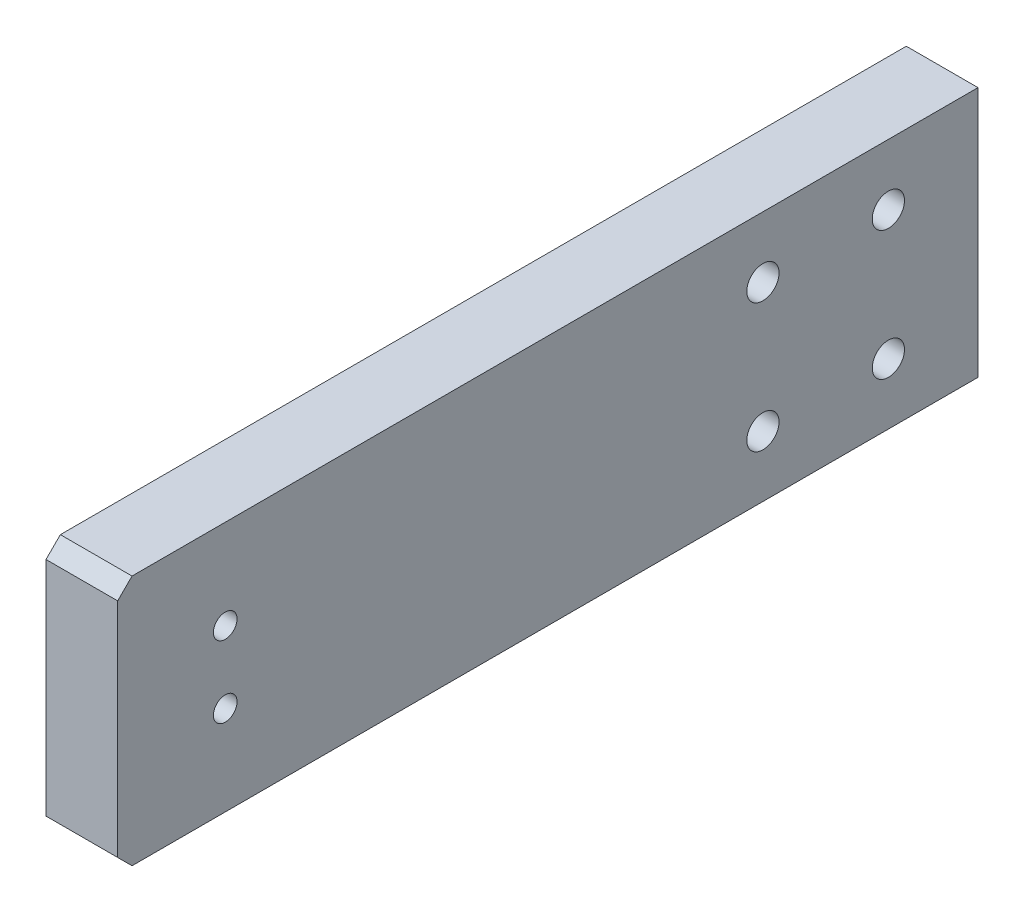
from build123d import *

# Parameters (mm, degrees)
SKETCH_1_W             = 120
SKETCH_1_H             = 35
EXTRUDE_1_DEPTH        = 10
HOLE_WIZARD_M4_1_D     = 3.3
SKETCH_5_R             = 2.25
CUT_EXTRUDE_1_DEPTH    = 28
CHAMFER_1_SIZE         = 2
PATTERN_LINEAR_1_COUNT = 2
PATTERN_LINEAR_1_PITCH = 17.5


with BuildPart() as part:
    # 草图1 → 凸台-拉伸1 (new body)
    with BuildSketch(Plane(origin=(0, 0, 0), x_dir=(0, 0, -1), z_dir=(1, 0, 0))):
        Rectangle(SKETCH_1_W, SKETCH_1_H)
    extrude(amount=EXTRUDE_1_DEPTH)

    # M4 螺纹孔1 (through all)
    with Locations(Plane.ZY):
        with Locations((45, 5), (45, -5)):
            Hole(HOLE_WIZARD_M4_1_D / 2)

    # 草图5 → 切除-拉伸1 (cut)
    with BuildSketch(Plane.ZY):
        with Locations((-47.5, 9)):
            Circle(SKETCH_5_R)
        with Locations(Location((-47.5, -9, 0), (0, 0, 180))):
            Circle(SKETCH_5_R)
    cut_extrude_1 = extrude(amount=-CUT_EXTRUDE_1_DEPTH, mode=Mode.SUBTRACT)

    # 倒角1
    chamfer_1_edges = [part.edges().sort_by_distance(p)[0] for p in [
        (5, -17.5, 60),
        (5, 17.5, 60),
    ]]
    chamfer(chamfer_1_edges, length=CHAMFER_1_SIZE)

    # 阵列(线性)1: 切除-拉伸1 ×2
    with Locations(*[(0, 0, i * PATTERN_LINEAR_1_PITCH) for i in range(1, PATTERN_LINEAR_1_COUNT)]):
        add(cut_extrude_1, mode=Mode.SUBTRACT)


solid = part.part
